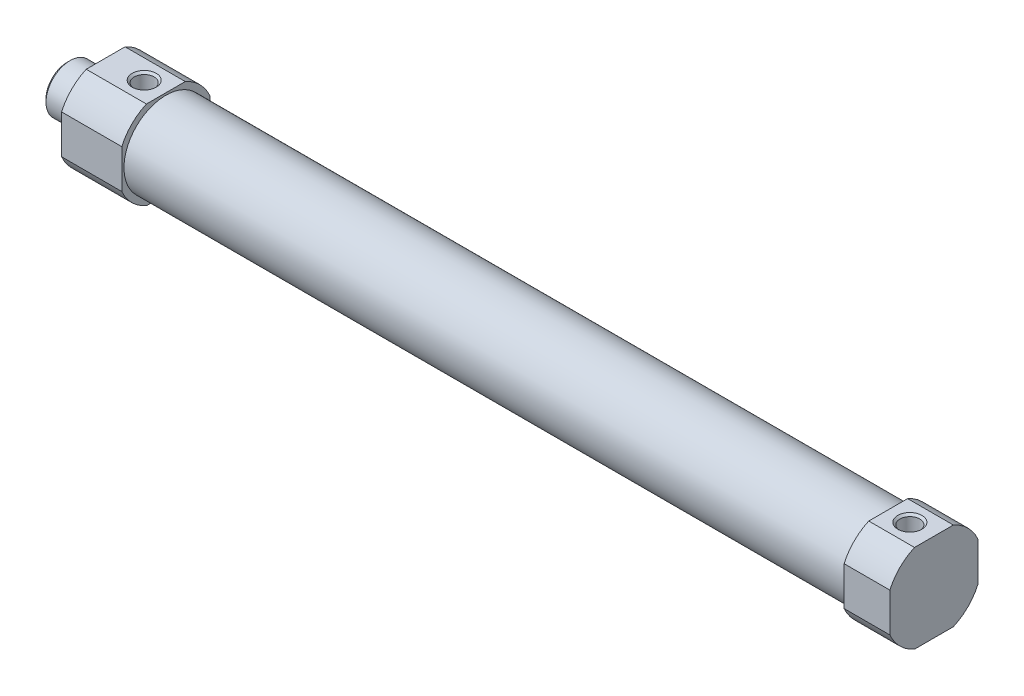
from build123d import *

# Parameters (mm, degrees)
BOSS_EXTRUDE1_DEPTH = 12.5
SKETCH3_R           = 8.7
BOSS_EXTRUDE2_DEPTH = 150
BOSS_EXTRUDE3_DEPTH = 9.5
HOLE1_D             = 4.134
HOLE1_DEPTH         = 5
HOLE1_CSINK_D       = 5
HOLE1_CSINK_ANGLE   = 90
HOLE1_TIP           = 1.193383006
HOLE2_D             = 4.134
HOLE2_DEPTH         = 5
HOLE2_CSINK_D       = 5
HOLE2_CSINK_ANGLE   = 90
HOLE2_TIP           = 1.193383006


with BuildPart() as part:
    # Sketch1 → Revolve1 (revolve)
    with BuildSketch(Plane.XY, mode=Mode.PRIVATE) as revolve1_sk:
        Polygon((-8, 0), (-8, 4.3865), (-7.3865, 5), (0, 5), (0, 0), align=None)
    revolve(revolve1_sk.sketch.rotate(Axis((0, 0, 0), (-1, 0, 0)), 270), axis=Axis((0, 0, 0), (-1, 0, 0)))

    # Sketch2 → Boss-Extrude1 (add)
    with BuildSketch(Plane(origin=(0, 0, 0), x_dir=(0, 0, -1), z_dir=(1, 0, 0))):
        with BuildLine():
            Line((-4.034538387, -9.15), (4.034538387, -9.15))
            ThreePointArc((4.034538387, -9.15), (7.071067812, -7.071067812), (9.15, -4.034538387))
            Line((9.15, -4.034538387), (9.15, 4.034538387))
            ThreePointArc((9.15, 4.034538387), (7.071067812, 7.071067812), (4.034538387, 9.15))
            Line((4.034538387, 9.15), (-4.034538387, 9.15))
            ThreePointArc((-4.034538387, 9.15), (-7.071067812, 7.071067812), (-9.15, 4.034538387))
            Line((-9.15, 4.034538387), (-9.15, -4.034538387))
            ThreePointArc((-9.15, -4.034538387), (-7.071067812, -7.071067812), (-4.034538387, -9.15))
        make_face()
    extrude(amount=BOSS_EXTRUDE1_DEPTH)

    # Sketch3 → Boss-Extrude2 (add)
    with BuildSketch(Plane(origin=(12.5, 0, 0), x_dir=(0, 0, -1), z_dir=(1, 0, 0))):
        Circle(SKETCH3_R)
    extrude(amount=BOSS_EXTRUDE2_DEPTH)

    # Sketch4 → Boss-Extrude3 (add)
    with BuildSketch(Plane(origin=(162.5, 0, 0), x_dir=(0, 0, -1), z_dir=(1, 0, 0))):
        with BuildLine():
            Line((-4.034538387, -9.15), (4.034538387, -9.15))
            ThreePointArc((4.034538387, -9.15), (7.071067812, -7.071067812), (9.15, -4.034538387))
            Line((9.15, -4.034538387), (9.15, 4.034538387))
            ThreePointArc((9.15, 4.034538387), (7.071067812, 7.071067812), (4.034538387, 9.15))
            Line((4.034538387, 9.15), (-4.034538387, 9.15))
            ThreePointArc((-4.034538387, 9.15), (-7.071067812, 7.071067812), (-9.15, 4.034538387))
            Line((-9.15, 4.034538387), (-9.15, -4.034538387))
            ThreePointArc((-9.15, -4.034538387), (-7.071067812, -7.071067812), (-4.034538387, -9.15))
        make_face()
    extrude(amount=BOSS_EXTRUDE3_DEPTH)

    # Hole1
    with Locations(Plane(origin=(0, 9.15, 0), x_dir=(1, 0, 0), z_dir=(0, 1, 0))):
        with Locations((8, 0)):
            CounterSinkHole(HOLE1_D / 2, HOLE1_CSINK_D / 2, depth=HOLE1_DEPTH, counter_sink_angle=HOLE1_CSINK_ANGLE)
            with Locations((0, 0, -(HOLE1_DEPTH + HOLE1_TIP / 2))):  # 120° drill point
                Cone(0, HOLE1_D / 2, HOLE1_TIP, mode=Mode.SUBTRACT)

    # Hole2
    with Locations(Plane(origin=(0, 9.15, 0), x_dir=(1, 0, 0), z_dir=(0, 1, 0))):
        with Locations((167, 0)):
            CounterSinkHole(HOLE2_D / 2, HOLE2_CSINK_D / 2, depth=HOLE2_DEPTH, counter_sink_angle=HOLE2_CSINK_ANGLE)
            with Locations((0, 0, -(HOLE2_DEPTH + HOLE2_TIP / 2))):  # 120° drill point
                Cone(0, HOLE2_D / 2, HOLE2_TIP, mode=Mode.SUBTRACT)

    # Sketch9 → Cut-Revolve1 (revolve, cut)
    with BuildSketch(Plane.XY, mode=Mode.PRIVATE) as cut_revolve1_sk:
        Polygon((-8, 0), (-8, 2.5), (12.5, 2.5), (12.5, 8), (142.5, 8), (142.5, 0), align=None)
    revolve(cut_revolve1_sk.sketch.rotate(Axis((50, 0, 0), (-1, 0, 0)), 270), axis=Axis((50, 0, 0), (-1, 0, 0)), mode=Mode.SUBTRACT)


solid = part.part
